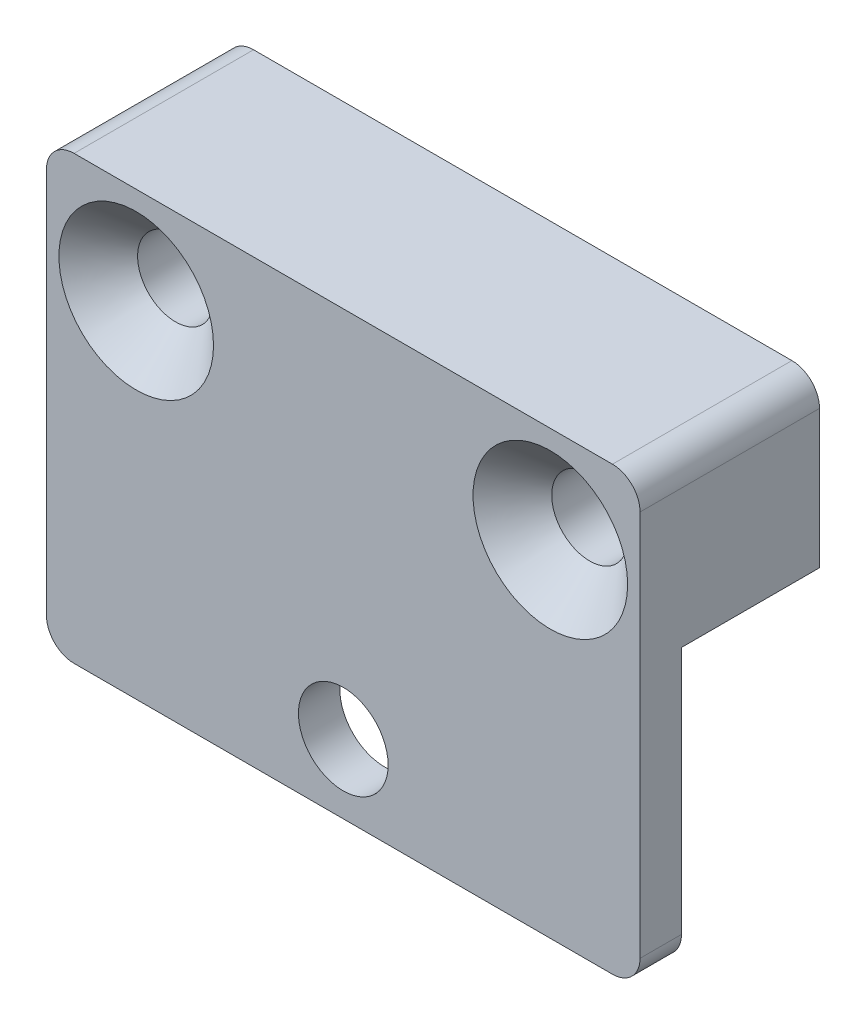
from build123d import *

# Parameters (mm, degrees)
SKETCH_1_W                  = 43
SKETCH_1_H                  = 32
EXTRUDE_1_DEPTH             = 3
HOLE_WIZARD_M5_1_AT_2_COUNT = 2
HOLE_WIZARD_M5_1_AT_2_PITCH = 30
SKETCH_4_R                  = 3.25
CUT_EXTRUDE_1_DEPTH         = 3
FILLET_1_R                  = 2
SKETCH_5_R                  = 2.75
EXTRUDE_2_DEPTH             = 10


with BuildPart() as part:
    # 草图1 → 凸台-拉伸1 (new body)
    with BuildSketch(Plane.XY):
        with Locations((21.5, -16)):
            Rectangle(SKETCH_1_W, SKETCH_1_H)
    extrude(amount=EXTRUDE_1_DEPTH)

    # 草图2 → M5 六角凹锥坑螺钉的锥形沉头孔1 (revolve, cut)
    with BuildSketch(Plane(origin=(6.5, -7, 3), x_dir=(0, -1, 0), z_dir=(1, 0, 0))):
        Polygon((0, 0), (0, 3), (2.75, 3), (2.75, 2.85), (5.6, 0), align=None)
    hole_wizard_m5_1 = revolve(axis=Axis((6.5, -7, 9.35), (0, 0, -1)), mode=Mode.SUBTRACT)

    # M5 六角凹锥坑螺钉的锥形沉头孔1 at 2: M5 六角凹锥坑螺钉的锥形沉头孔1 ×2
    with Locations(*[(i * HOLE_WIZARD_M5_1_AT_2_PITCH, 0, 0) for i in range(1, HOLE_WIZARD_M5_1_AT_2_COUNT)]):
        add(hole_wizard_m5_1, mode=Mode.SUBTRACT)

    # 草图4 → 切除-拉伸1 (cut)
    with BuildSketch(Plane.XY.offset(3)):
        with Locations((21.5, -27)):
            Circle(SKETCH_4_R)
    extrude(amount=-CUT_EXTRUDE_1_DEPTH, mode=Mode.SUBTRACT)

    # 圆角1
    fillet_1_edges = [part.edges().sort_by_distance(p)[0] for p in [
        (0, 0, 1.5),
        (43, 0, 1.5),
        (43, -32, 1.5),
        (0, -32, 1.5),
    ]]
    fillet(fillet_1_edges, radius=FILLET_1_R)

    # 草图5 → 凸台-拉伸2 (add)
    with BuildSketch(Plane(origin=(0, 0, 0), x_dir=(-1, 0, 0), z_dir=(0, 0, -1))):
        with BuildLine():
            Line((-43, -2), (-43, -12))
            Line((-43, -12), (0, -12))
            Line((0, -12), (0, -2))
            ThreePointArc((0, -2), (-0.585786438, -0.585786438), (-2, 0))
            Line((-2, 0), (-41, 0))
            ThreePointArc((-41, 0), (-42.414213562, -0.585786438), (-43, -2))
        make_face()
        with Locations(Location((-36.5, -7, 0), (0, 0, 180))):
            Circle(SKETCH_5_R, mode=Mode.SUBTRACT)
        with Locations(Location((-6.5, -7, 0), (0, 0, 180))):
            Circle(SKETCH_5_R, mode=Mode.SUBTRACT)
    extrude(amount=EXTRUDE_2_DEPTH)


solid = part.part
